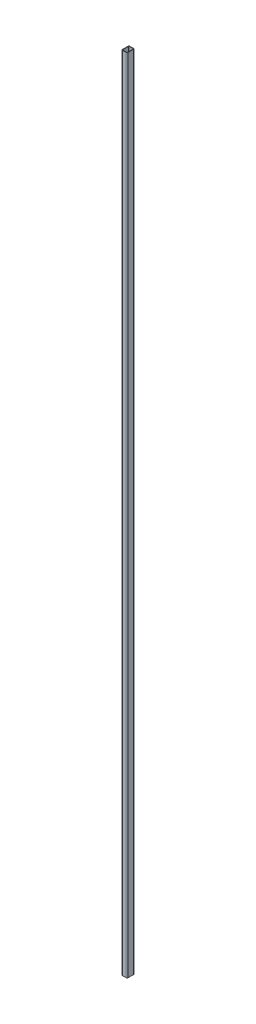
from build123d import *

# Parameters (mm, degrees)
COLD_FORMED_HOLLOW_RECTANGULAR_STEEL_GB_DEPTH = 8850


with BuildPart() as part:
    # Sketch1 → Cold-formed hollow rectangular steel (GB/T 6728-2002) 80×60×5(1) (new body)
    with BuildSketch(Plane(origin=(0, 0, 0), x_dir=(-1, 0, 0), z_dir=(0, 1, 0))):
        with BuildLine():
            Line((-20, -40), (20, -40))
            ThreePointArc((20, -40), (27.071067812, -37.071067812), (30, -30))
            Line((30, -30), (30, 30))
            ThreePointArc((30, 30), (27.071067812, 37.071067812), (20, 40))
            Line((20, 40), (-20, 40))
            ThreePointArc((-20, 40), (-27.071067812, 37.071067812), (-30, 30))
            Line((-30, 30), (-30, -30))
            ThreePointArc((-30, -30), (-27.071067812, -37.071067812), (-20, -40))
        make_face()
        with BuildLine():
            Line((-20, -35), (20, -35))
            ThreePointArc((20, -35), (23.535533906, -33.535533906), (25, -30))
            Line((25, -30), (25, 30))
            ThreePointArc((25, 30), (23.535533906, 33.535533906), (20, 35))
            Line((20, 35), (-20, 35))
            ThreePointArc((-20, 35), (-23.535533906, 33.535533906), (-25, 30))
            Line((-25, 30), (-25, -30))
            ThreePointArc((-25, -30), (-23.535533906, -33.535533906), (-20, -35))
        make_face(mode=Mode.SUBTRACT)
    extrude(amount=COLD_FORMED_HOLLOW_RECTANGULAR_STEEL_GB_DEPTH)


solid = part.part
